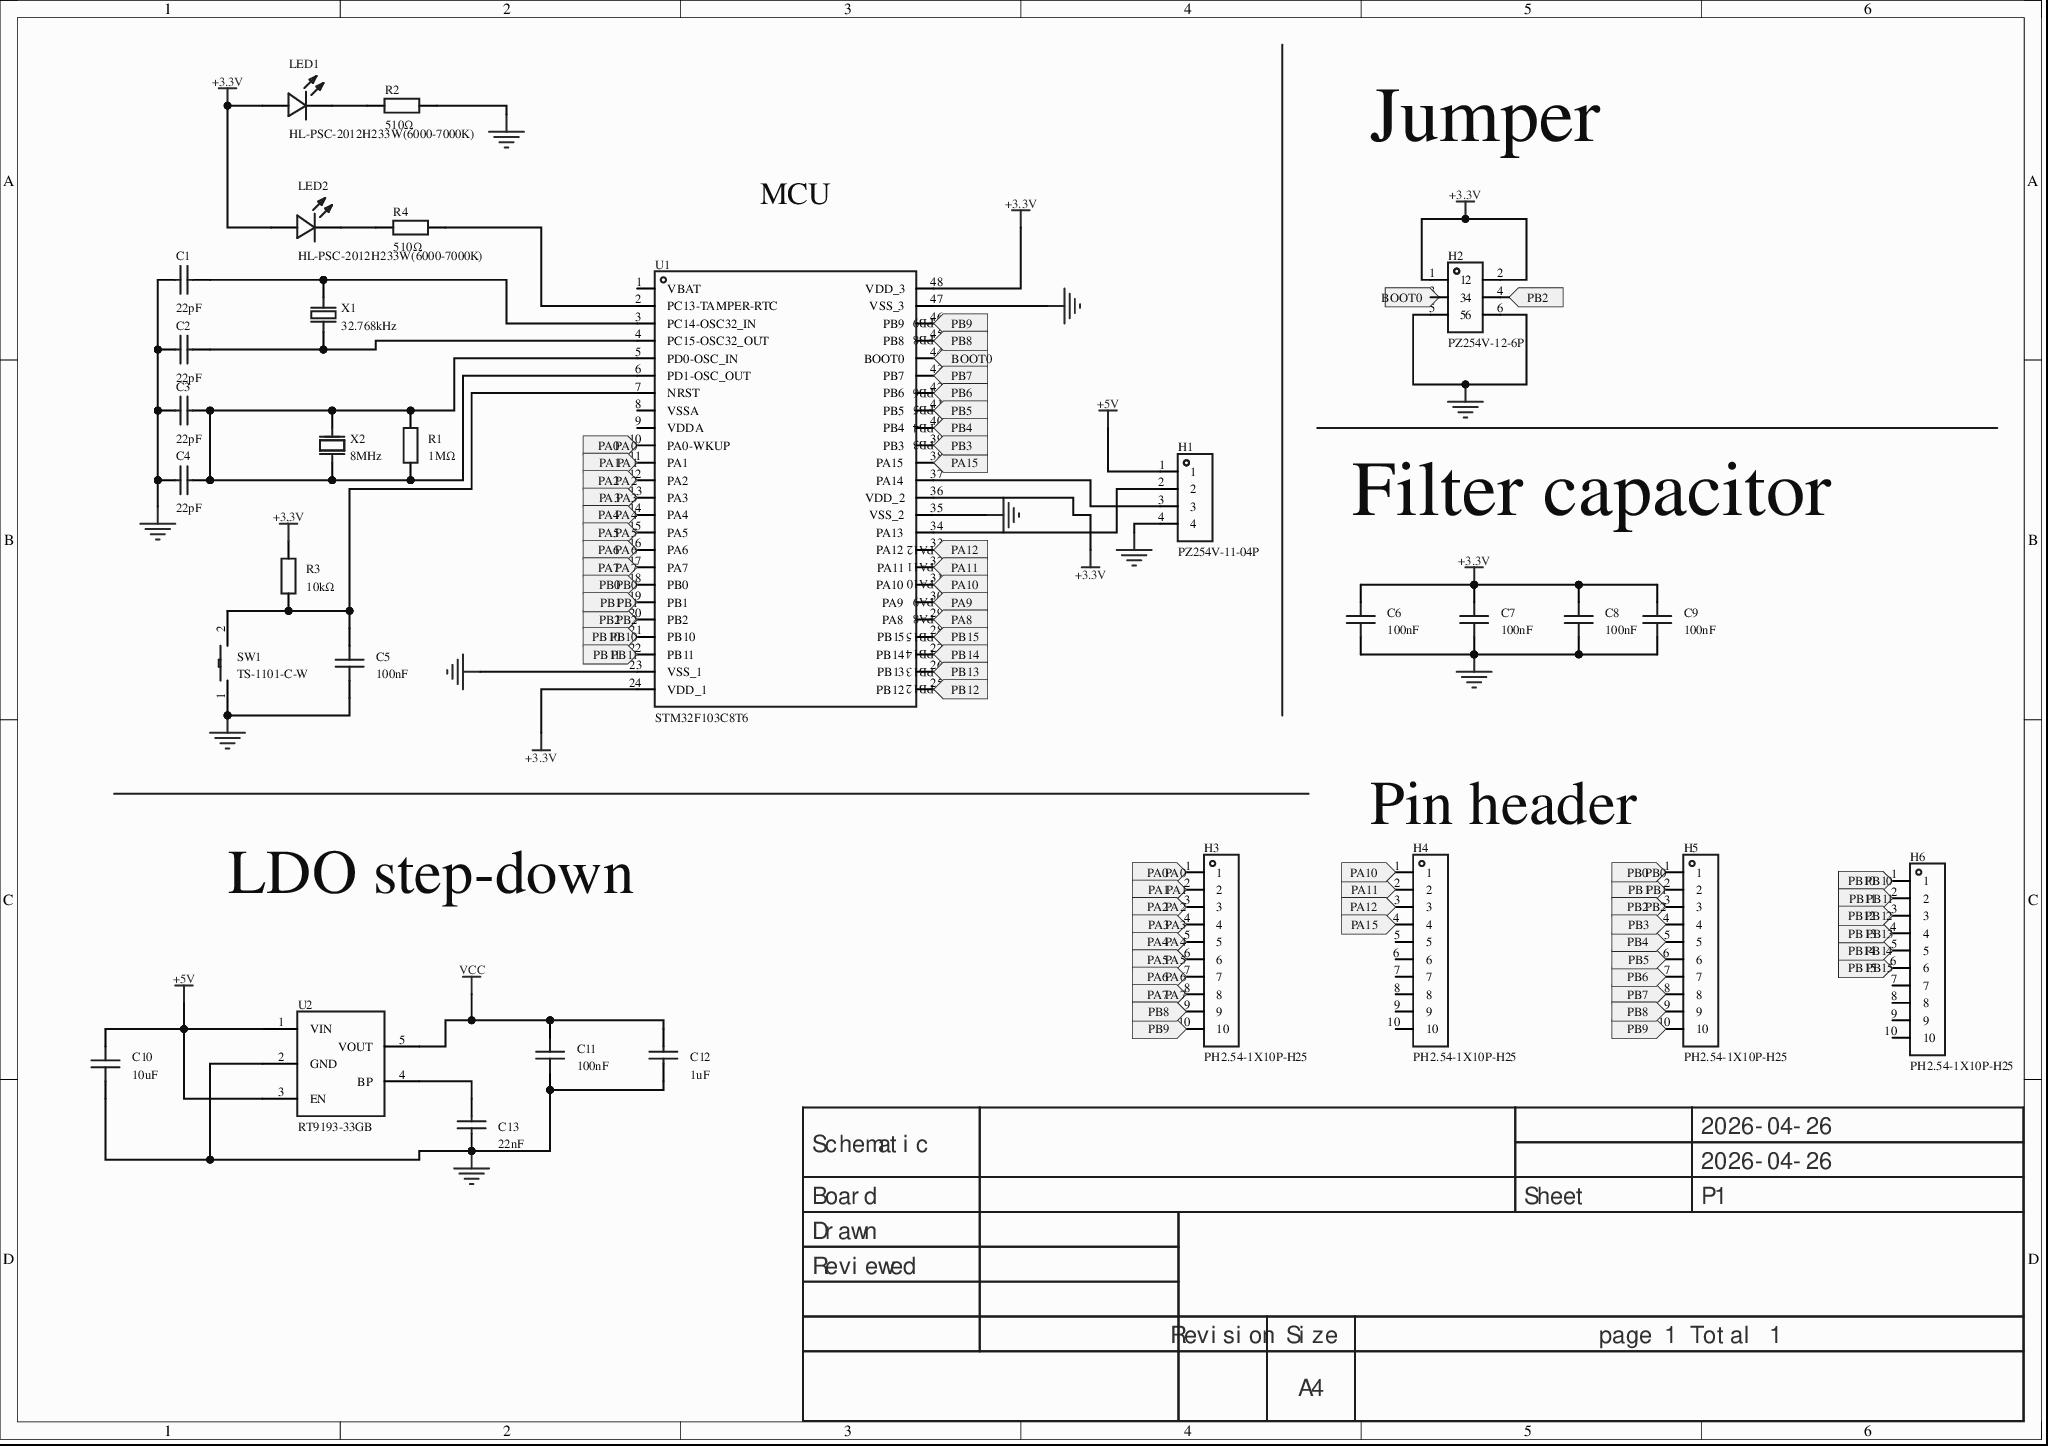
[diagram p0: MISC52025-3.schdoc]
# Altium project MISC52025-2.PrjPcb
1 sheet, 30 parts. Net scope: flat (ports and power ports of the same name join across sheets).
Board file: MISC52025.pcbdoc

## Sheet MISC52025-3.schdoc
size 297 x 209 mm; Version: V1.0; @Project Name: MISC52025; @Update Date: 2026-04-26; @Create Date: 2026-04-26; @Board Name: MISC52025; @Create Time: 15:19:25; @Page Count: 1; @Page No: 1; @Schematic Name: MISC52025; @Update Time: 15:19:25; Size: A4

### Parts
C1  22pF  [C0603]
C2  22pF  [C0603]
C3  22pF  [C0603]
C4  22pF  [C0603]
C5  100nF  [C0603]
C6  100nF  [C0603]
C7  100nF  [C0603]
C8  100nF  [C0603]
C9  100nF  [C0603]
C10  10uF  [C0603]
C11  100nF  [C0603]
C12  1uF  [C0603]
C13  22nF  [C0603]
H1  PZ254V-11-04P  [HDR-TH_4P-P2.54-V-M]
H2  PZ254V-12-6P  [HDR-TH_6P-P2.54-V-M-R2-C3-S2.54]
H3  PH2.54-1X10P-H25  [HDR-TH_10P-P2.54-V-M]
H4  PH2.54-1X10P-H25  [HDR-TH_10P-P2.54-V-M]
H5  PH2.54-1X10P-H25  [HDR-TH_10P-P2.54-V-M]
H6  PH2.54-1X10P-H25  [HDR-TH_10P-P2.54-V-M]
LED1  HL-PSC-2012H233W(6000-7000K)  [LED0805-R-RD]
LED2  HL-PSC-2012H233W(6000-7000K)  [LED0805-R-RD]
R1  1MΩ  [R0805]
R2  510Ω  [R0603]
R3  10kΩ  [R0603]
R4  510Ω  [R0603]
SW1  TS-1101-C-W  [SW-SMD_L6.0-W3.3-LS8.0_TS-1101-C-W]
U1  STM32F103C8T6  [LQFP-48_L7.0-W7.0-P0.50-LS9.0-BL]
U2  RT9193-33GB  [SOT-23-5_L3.0-W1.7-P0.95-LS2.8-BL]
X1  32.768kHz  [FC-135R_L3.2-W1.5]
X2  8MHz  [CRYSTAL-SMD_L5.0-W3.2]

### Ports
BOOT0 (in), PA0 (in), PA1 (in), PA2 (in), PA3 (in), PA4 (in), PA5 (in), PA6 (in), PA7 (in), PA8 (in), PA9 (in), PA10 (in), PA11 (in), PA12 (in), PA15 (in), PB0 (in), PB1 (in), PB2 (in), PB3 (in), PB4 (in), PB5 (in), PB6 (in), PB7 (in), PB8 (in), PB9 (in), PB10 (in), PB11 (in), PB12 (in), PB13 (in), PB14 (in), PB15 (in)

### Nets
+3,3V: R3.2
+3.3V: C6.2 C7.2 C8.2 C9.2 H2.1 H2.2 LED1.1(A) LED2.1(A) U1.24(VDD_1) U1.36(VDD_2) U1.48(VDD_3)
+5V: C10.2 H1.1 U2.1(VIN) U2.3(EN)
GND: C1.1 C2.1 C3.1 C4.1 C5.1 C6.1 C7.1 C8.1 C9.1 C10.1 C11.1 C12.1 C13.1 H1.4 H2.5 H2.6 R2.2 SW1.1 U1.23(VSS_1) U1.35(VSS_2) U1.47(VSS_3) U2.2(GND)
VCC: C11.2 C12.2 U2.5(VOUT)
PA0: H3.1 U1.10(PA0-WKUP) ; port PA0
PA1: H3.2 U1.11(PA1) ; port PA1
PA2: H3.3 U1.12(PA2) ; port PA2
PA3: H3.4 U1.13(PA3) ; port PA3
PA4: H3.5 U1.14(PA4) ; port PA4
PA5: H3.6 U1.15(PA5) ; port PA5
PA6: H3.7 U1.16(PA6) ; port PA6
PA7: H3.8 U1.17(PA7) ; port PA7
PA8: U1.29(PA8) ; port PA8
PA9: U1.30(PA9) ; port PA9
PA10: H4.1 U1.31(PA10) ; port PA10
PA11: H4.2 U1.32(PA11) ; port PA11
PA12: H4.3 U1.33(PA12) ; port PA12
PB0: H5.1 U1.18(PB0) ; port PB0
PB1: H5.2 U1.19(PB1) ; port PB1
PB2: H2.4 H5.3 U1.20(PB2) ; port PB2
PB3: H5.4 U1.39(PB3) ; port PB3
PB4: H5.5 U1.40(PB4) ; port PB4
PB5: H5.6 U1.41(PB5) ; port PB5
PB6: H5.7 U1.42(PB6) ; port PB6
PB8: H3.9 H5.9 U1.45(PB8) ; port PB8
PB9: H3.10 H5.10 U1.46(PB9) ; port PB9
PB10: H6.1 U1.21(PB10) ; port PB10
PB11: H6.2 U1.22(PB11) ; port PB11
PB12: H6.3 U1.25(PB12) ; port PB12
PB13: H6.4 U1.26(PB13) ; port PB13
PB14: H6.5 U1.27(PB14) ; port PB14
PB15: H6.6 U1.28(PB15) ; port PB15
NetC1_2: C1.2 U1.3(PC14-OSC32_IN) X1.2
NetC2_2: C2.2 U1.4(PC15-OSC32_OUT) X1.1
NetC3_2: C3.2 C4.2 R1.1 R1.2 U1.5(PD0-OSC_IN) U1.6(PD1-OSC_OUT) X2.1(OSC1) X2.2(OSC2)
NetC5_2: C5.2 R3.1 SW1.2 U1.7(NRST)
NetC13_2: C13.2 U2.4(BP)
NetH1_2: H1.2 U1.34(PA13)
NetH1_3: H1.3 U1.37(PA14)
NetH2_3: H2.3 U1.44(BOOT0) ; port BOOT0
NetH4_4: H4.4 U1.38(PA15) ; port PA15
NetH5_8: H5.8 U1.43(PB7) ; port PB7
NetLED1_2: LED1.2(C) R2.1
NetLED2_2: LED2.2(C) R4.1
NetR4_2: R4.2 U1.2(PC13-TAMPER-RTC)

Not connected (* = marked no-connect by the designer): H4 5 6 7 8 9 10; H6 7 8 9 10; U1 1(VBAT) 8(VSSA) 9(VDDA)

### Notes on the sheet
- Jumper
- MCU
- Filter capacitor
- Pin header
- LDO step-down
- 2026-04-26
- Schematic
- Board
- Sheet
- P1
- Drawn
- Reviewed
- Revision
- Size
- A4
- page 1 Total 1

### Library data of the parts
C1-C4 = CL10C220JB8NNNC: Capacitance:22pF;Tolerance:±5%;Rated voltage:50V;Temperature coefficient:C0G;; Manufacturer: SAMSUNG(三星); 3D Model: ac125912035d415993ca9572d50418b10819f05c4eef4c71ace90d822a990e87; 3D Model Transform: 62.992,31.496,0,0,0,0,0,0,0; Tolerance: ±5%; Voltage Rating: 50V; Temperature Coefficient: C0G; AddInBom: yes; ModelName: C0603_L1.6-W0.8-H0.8; Symbol: CL10C220JB8NNNC; Device: CL10C220JB8NNNC; LCSC Part Name: 22pF ±5% 50V; Supplier Part: C1653; Manufacturer Part: CL10C220JB8NNNC; Supplier Footprint: 0603; JLCPCB Part Class: Basic Part; Datasheet: https://example.com/datasheet/CL10C220JB8NNNC/2005.html; Supplier: LCSC; Value: 22pF; ConvertToPcb: yes; FootprintName: C0603
C5-C9 C11 = CC0603KRX7R9BB104: Capacitance:100nF;Tolerance:±10%;Rated voltage:50V;Temperature coefficient:X7R;; Manufacturer: YAGEO(国巨); AddInBom: yes; ModelId: ac125912035d415993ca9572d50418b10819f05c4eef4c71ace90d822a990e87; ModelName: C0603_L1.6-W0.8-H0.8; ModelTransform: 62.992,31.496,0,0,0,0,0,0,0; Tolerance: ±10%; Voltage Rating: 50V; Temperature Coefficient: X7R; Symbol: CC0603KRX7R9BB104; Device: CC0603KRX7R9BB104; LCSC Part Name: 100nF ±10% 50V; SupplierPart: C14663; ManufacturerPart: CC0603KRX7R9BB104; Supplier Footprint: 0603; JLCPCB Part Class: Basic Part; Datasheet: https://example.com/datasheet/CC0603KRX7R9BB104/15331.html; Supplier: LCSC; ConvertToPcb: yes; FootprintName: C0603; Value: 100nF
C10 = CL10A106KP8NNNC: Capacitance:10uF;Tolerance:±10%;Rated voltage:10V;Temperature coefficient:X5R;; Manufacturer: SAMSUNG(三星); AddInBom: yes; ModelId: ac125912035d415993ca9572d50418b10819f05c4eef4c71ace90d822a990e87; ModelName: C0603_L1.6-W0.8-H0.8; ModelTransform: 62.992,31.496,0,0,0,0,0,0,0; Tolerance: ±10%; Voltage Rating: 10V; Temperature Coefficient: X5R; Symbol: CL10A106KP8NNNC; Device: CL10A106KP8NNNC; LCSC Part Name: 10uF ±10% 10V; SupplierPart: C19702; ManufacturerPart: CL10A106KP8NNNC; Supplier Footprint: 0603; JLCPCB Part Class: Basic Part; Datasheet: https://example.com/datasheet/CL10A106KP8NNNC/20411.html; Supplier: LCSC; ConvertToPcb: yes; FootprintName: C0603; Value: 10uF
C12 = CL10B105KO8NNNC: Capacitance:1uF;Tolerance:±10%;Rated voltage:16V;Temperature coefficient:X7R;; Manufacturer: SAMSUNG(三星); AddInBom: yes; ModelId: ac125912035d415993ca9572d50418b10819f05c4eef4c71ace90d822a990e87; ModelName: C0603_L1.6-W0.8-H0.8; ModelTransform: 62.992,31.496,0,0,0,0,0,0,0; Tolerance: ±10%; Voltage Rating: 16V; Temperature Coefficient: X7R; Symbol: CL10B105KO8NNNC; Device: CL10B105KO8NNNC; LCSC Part Name: 1uF ±10% 16V; SupplierPart: C59782; ManufacturerPart: CL10B105KO8NNNC; Supplier Footprint: 0603; JLCPCB Part Class: Extended Part; Datasheet: https://example.com/datasheet/CL10B105KO8NNNC/60834.html; Supplier: LCSC; ConvertToPcb: yes; FootprintName: C0603; Value: 1uF
C13 = CL10B223KB8NNNC: Capacitance:22nF;Tolerance:±10%;Rated voltage:50V;Temperature coefficient:X7R;; Manufacturer: SAMSUNG(三星); AddInBom: yes; ModelId: ac125912035d415993ca9572d50418b10819f05c4eef4c71ace90d822a990e87; ModelName: C0603_L1.6-W0.8-H0.8; ModelTransform: 62.992,31.496,0,0,0,0,0,0,0; Tolerance: ±10%; Voltage Rating: 50V; Temperature Coefficient: X7R; Symbol: CL10B223KB8NNNC; Device: CL10B223KB8NNNC; LCSC Part Name: 22nF ±10% 50V; SupplierPart: C21122; ManufacturerPart: CL10B223KB8NNNC; Supplier Footprint: 0603; JLCPCB Part Class: Basic Part; Datasheet: https://example.com/datasheet/CL10B223KB8NNNC/21834.html; Supplier: LCSC; ConvertToPcb: yes; FootprintName: C0603; Value: 22nF
H1 = PZ254V-11-04P: Pin structure:1x4P;Pitch:2.54mm;Row spacing:-;Round/square pin:Square;Mounting:Through-hole;Rows:Single row;Total pins:4P;Rated current:3A;Rated voltage:250V;Mating pin length:6mm;Housing height:2.5mm;Termination pin length:3mm;Contact material:-;Operating temperature:-40℃~+105℃;Colour:Black;; Manufacturer: XFCN(兴飞); Symbol: PZ254V-11-04P_C2691448; AddInBom: yes; ModelId: 112f4d05e8d64e99ab9a333894bea4f90819f05c4eef4c71ace90d822a990e87; ModelName: HDR-TH_4P-P2.54-M-LI-1X4P; ModelTransform: 399.999,104.7242,0,0,0,0,0,0,-118.11; Pin Structure: 1x4P; Pitch: 2.54mm; Circluar Pins/Square Pins: Square; Current Rating: 3A; Voltage Rating (Max): 250V; Device: PZ254V-11-04P; LCSC Part Name: 1x4P 间距:2.54mm 方针 直插; SupplierPart: C2691448; ManufacturerPart: PZ254V-11-04P; Supplier Footprint: 插件,P=2.54mm; JLCPCB Part Class: Extended Part; Datasheet: https://example.com/datasheet/PZ254V-11-04P/2801085.html; Supplier: LCSC; ConvertToPcb: yes; FootprintName: HDR-TH_4P-P2.54-V-M; Row Spacing: -; Mounting Type: Through-hole; Number of Rows: Single row; Number of Pins: 4P; Length of Mating Pin: 6mm; Insulation Height: 2.5mm; Length of End Connection Pin: 3mm; Contact Material: -; Operating Temperature: -40℃~+105℃; Color: Black
H2 = PZ254V-12-6P: Pin structure:2x3P;Pitch:2.54mm;Row spacing:2.54mm;Round/square pin:Square;Mounting type:Through-hole;Rows:Dual row;Total pins:6P;Rated current:-;Rated voltage:-;Mating pin length:6mm;Housing height:2.5mm;Termination pin length:3mm;Contact material:Brass;Contact plating:-;Operating temperature range:-40℃~+105℃;Colour:Black;; Manufacturer: XFCN(兴飞); AddInBom: yes; ModelId: e22692306cbd4b5c8488f4142eed6b9c0819f05c4eef4c71ace90d822a990e87; ModelTransform: 300.3931,200,0,0,0,0,0,0,-118.11; Pin Structure: 2x3P; Pitch: 2.54mm; Circluar Pins/Square Pins: Square; Symbol: PZ254V-12-6P; Device: PZ254V-12-6P; LCSC Part Name: 间距:2.54mm 2x3P 直插 方针; SupplierPart: C492420; ManufacturerPart: PZ254V-12-6P; Supplier Footprint: 插件,P=2.54mm; JLCPCB Part Class: Extended Part; Datasheet: https://example.com/upload/public/pdf/source/20200309/C492420_BAECB307B001054C09D200388220EAE6.pdf; Supplier: LCSC; ConvertToPcb: yes; FootprintName: HDR-TH_6P-P2.54-V-M-R2-C3-S2.54; ModelName: HDR-TH_6P-P2.54-V-M-R2-C3-S2.54; Row Spacing: 2.54mm; Mounting Type: Through-hole; Number of Rows: Dual row; Number of Pins: 6P; Current Rating (Max): -; Voltage Rating (Max): -; Length of Mating Pin: 6mm; Insulation Height: 2.5mm; Length of End Connection Pin: 3mm; Contact Material: Brass; Contact Plating: -; Operating Temperature Range: -40℃~+105℃; Color: Black
H3-H6 = PH2.54-1X10P-H25: Pin structure:1x10P;Pitch:2.54mm;Row spacing:-;Round/square pin:Square;Mounting:Through-hole;Rows:Single row;Total pins:10P;Rated current:3A;Rated voltage:-;Mating pin length:6mm;Housing height:2.5mm;Termination pin length:3mm;Contact material:Brass;Contact plating:Gold;Operating temperature:-40℃~+105℃;Colour:Black;; Manufacturer: JXTCONN(聚兴泰); AddInBom: yes; ModelId: 10f3d1cea59e4bb4ba116af9f09c2b9b0819f05c4eef4c71ace90d822a990e87; ModelName: HDR2.54-M-LI-1X10P; ModelTransform: 999.99796,100,0,0,0,0,0,0,-118.11; Pin Structure: 1x10P; Pitch: 2.54mm; Circluar Pins/Square Pins: Square; Current Rating: 3A; Symbol: PH2.54-1X10P-H25; Device: PH2.54-1X10P-H25; LCSC Part Name: 1x10P 间距:2.54mm 方针 直插; SupplierPart: C42431810; ManufacturerPart: PH2.54-1X10P-H25; Supplier Footprint: 插件,P=2.54mm; JLCPCB Part Class: Extended Part; Datasheet: https://example.com/datasheet/PH2.54-1X10P-H25/44458940.html; Supplier: LCSC; ConvertToPcb: yes; FootprintName: HDR-TH_10P-P2.54-V-M; Row Spacing: -; Mounting Type: Through-hole; Number of Rows: Single row; Number of Pins: 10P; Voltage Rating (Max): -; Length of Mating Pin: 6mm; Insulation Height: 2.5mm; Length of End Connection Pin: 3mm; Contact Material: Brass; Contact Plating: Gold; Operating Temperature: -40℃~+105℃; Color: Black
LED1 LED2 = HL-PSC-2012H233W(6000-7000K): Lamp base type:-;Emitting colour:White;Forward voltage (Vf):3.4V;Power:102mW;Forward current:20mA;Wavelength:-;Diode configuration:Single diode;Lens colour:Frosted yellow lens;Colour temperature:6000K~7000K;Luminous intensity:1.4cd;Viewing angle:140°;Tape packaging:Top mount;Operating temperature:-40℃~+85℃;; Manufacturer: HONGLITRONIC(鸿利光电); AddInBom: yes; ModelId: 6ccd75a2b5134d6ab756ecf3c14a72900819f05c4eef4c71ace90d822a990e87; ModelName: LED0805-RD; ModelTransform: 79.527,49.2125,0,0,0,0,0,0,0; Illumination Color: White; Voltage - Forward(Vf): 3.4V; Power(Watts): 102mW; Forward Current: 20mA; Luminous Intensity: 1.4cd; Viewing Angle: 140°; Symbol: HL-PSC-2012H233W(6000-7000K); Device: HL-PSC-2012H233W(6000-7000K); LCSC Part Name: 白色; SupplierPart: C219231; ManufacturerPart: HL-PSC-2012H233W(6000-7000K); Supplier Footprint: 0805; JLCPCB Part Class: Extended Part; Datasheet: https://example.com/datasheet/HL-PSC-2012H233W(6000-7000K)/220090.html; Supplier: LCSC; ConvertToPcb: yes; FootprintName: LED0805-R-RD; Lamp Holder Type: -; Wavelength - Dominant: -; Peak Wavelength: -; Diode Configuration: Single diode; Lens Color: Frosted yellow lens; Color Temperature: 6000K~7000K; Mounting Style: Top mount; Operating Temperature: -40℃~+85℃
R1 = 0805W8F1004T5E: Resistor type:Thick film resistor;Resistance:1MΩ;Tolerance:±1%;Power:125mW;Max working voltage:150V;Temperature coefficient:±100ppm/℃;; Manufacturer: UNI-ROYAL(厚声); AddInBom: yes; ModelId: 37a81e68749a4138bd2dfa6897b24b850819f05c4eef4c71ace90d822a990e87; ModelName: R0805_L2.0-W1.3-H0.6; ModelTransform: 78.74,51.181,0,0,0,0,0,-0.0005,0; Tolerance: ±1%; Power(Watts): 125mW; Overload Voltage (Max): 150V; Symbol: 0805W8F1004T5E; Device: 0805W8F1004T5E; LCSC Part Name: 1MΩ ±1% 125mW 厚膜电阻; SupplierPart: C17514; ManufacturerPart: 0805W8F1004T5E; Supplier Footprint: 0805; JLCPCB Part Class: Basic Part; Datasheet: https://example.com/upload/public/pdf/source/20200306/C422600_1E6D84923E4A46A82E41ADD87F860B5C.pdf; Supplier: LCSC; ConvertToPcb: yes; FootprintName: R0805; Type: Thick film resistor; Value: 1MΩ; Temperature Coefficient: ±100ppm/℃; Operating Temperature Range: -55℃~+155℃
R2 R4 = 0603WAF5100T5E: Resistor type:Thick film resistor;Resistance:510Ω;Tolerance:±1%;Power:100mW;Working voltage:75V;Temperature coefficient:±100ppm/℃;; Manufacturer: UNI-ROYAL(厚声); AddInBom: yes; ModelId: fc143cca1e79419f9cd78b61e9279f080819f05c4eef4c71ace90d822a990e87; ModelTransform: 31.8897,63.7794,0,90,0,0,0,0,0; Tolerance: ±1%; Power(Watts): 100mW; Voltage-Supply(Max): 75V; Symbol: 0603WAF5100T5E; Device: 0603WAF5100T5E; LCSC Part Name: 510Ω ±1% 100mW 厚膜电阻; SupplierPart: C23193; ManufacturerPart: 0603WAF5100T5E; Supplier Footprint: 0603; JLCPCB Part Class: Basic Part; Datasheet: https://example.com/datasheet/0603WAF5100T5E/23920.html; Supplier: LCSC; ConvertToPcb: yes; FootprintName: R0603; ModelName: R0603; Type: Thick film resistor; Value: 510Ω; Temperature Coefficient: ±100ppm/℃; Operating Temperature: -55℃~+155℃
R3 = 0603WAF1002T5E: Resistor type:Thick film resistor;Resistance:10kΩ;Tolerance:±1%;Power:100mW;Working voltage:75V;Temperature coefficient:±100ppm/℃;; Manufacturer: UNI-ROYAL(厚声); AddInBom: yes; ModelId: fc143cca1e79419f9cd78b61e9279f080819f05c4eef4c71ace90d822a990e87; ModelTransform: 31.8897,63.7794,0,90,0,0,0,0,0; Tolerance: ±1%; Power(Watts): 100mW; Voltage-Supply(Max): 75V; Symbol: 0603WAF1002T5E; Device: 0603WAF1002T5E; LCSC Part Name: 厚膜电阻 10kΩ ±1% 100mW; SupplierPart: C25804; ManufacturerPart: 0603WAF1002T5E; Supplier Footprint: 0603; JLCPCB Part Class: Basic Part; Datasheet: https://example.com/datasheet/0603WAF1002T5E/26547.html; Supplier: LCSC; ConvertToPcb: yes; FootprintName: R0603; ModelName: R0603; Type: Thick film resistor; Value: 10kΩ; Temperature Coefficient: ±100ppm/℃; Operating Temperature: -55℃~+155℃
SW1 = TS-1101-C-W: Circuit structure:SPST;Button shape:Rectangular button;Actuating force:2.6N;Mounting:Upright SMD;Switch length:6mm;Switch width:3.6mm;Switch height:2.5mm;Bracket:Without bracket;Contact current:50mA;Rated voltage:12V;Lamp:None;Life:5万 cycles;; Manufacturer: XKB Connection(中国星坤); AddInBom: yes; ModelId: 0fd6340cfb7d45bfbbb5f8576d023f850819f05c4eef4c71ace90d822a990e87; ModelTransform: 315.232,145.669,0,0,0,0,0,0,0; Circuit: SPST; Operating Force: 2.6N; Switch Height: 2.5mm; Contact Current: 50mA; Voltage Rating: 12V; With Lamp: None; Symbol: TS-1101-C-W; Device: TS-1101-C-W; LCSC Part Name: 6*3.6*2.5mm 立贴 轻触开关; SupplierPart: C318938; ManufacturerPart: TS-1101-C-W; Supplier Footprint: SMD,6x3.6mm; JLCPCB Part Class: Extended Part; Datasheet: https://example.com/datasheet/TS-1101-C-W/300030.html; Supplier: LCSC; ConvertToPcb: yes; FootprintName: SW-SMD_L6.0-W3.3-LS8.0_TS-1101-C-W; ModelName: SW-SMD_L6.0-W3.3-LS8.0_TS-1101-C-W; Actuator Style: Rectangular button; Mounting Type: Upright SMD; Length: 6mm; Width: 3.6mm; with Bracket: Without bracket; Actuator/Cap Color: -; IP Rating: -; Termination Style: -; Life: 5万 cycles; Operating Temperature: -30℃~+85℃
U1 = STM32F103C8T6: CPU core:ARM-M3;CPU max frequency:72MHz;Application field:-;; Manufacturer: ST(意法半导体); 3D Model: 093be70396ff421eb2cdb946d5311efc0819f05c4eef4c71ace90d822a990e87; 3D Model Transform: 354.331,354.331,0,0,0,0,0,0,0; CPU Core: ARM-M3; CPU Maximum Speed: 72MHz; Program Storage Size: 64KB; Program Memory Type: FLASH; Number of I/O: 37; ADC (Bit): 12bit; Voltage - Supply: 2V~3.6V; AddInBom: yes; ModelName: LQFP-48_L7.0-W7.0-H1.4-LS9.0-P0.50; Symbol: STM32F103C8T6; Device: STM32F103C8T6; LCSC Part Name: 主流增强型ARM Cortex-M3 MCU，具有64 KB Flash、72 MHz CPU、电机控制、USB和CAN; Supplier Part: C8734; Manufacturer Part: STM32F103C8T6; Supplier Footprint: LQFP-48(7x7); JLCPCB Part Class: Extended Part; Datasheet: https://example.com/datasheet/STM32F103C8T6/9243.html; Supplier: LCSC; Applications: -; ConvertToPcb: yes; FootprintName: LQFP-48_L7.0-W7.0-P0.50-LS9.0-BL
U2 = RT9193-33GB: Output type:Fixed;Working voltage:5.5V;Output voltage:3.3V;Output current:300mA;Power supply ripple rejection (PSRR):-50dB@(10kHz);Output polarity:Positive;; Manufacturer: RICHTEK(立锜); AddInBom: yes; ModelId: 0a2a1b8f50944f73965918ad6e5fe1670819f05c4eef4c71ace90d822a990e87; ModelName: SOT-23-5_L2.9-W1.6-H1.1-LS2.8-P0.95; ModelTransform: 118.60433,114.173,0,90,0,0,0.0005,0.0005,0; Output Type: Fixed; Voltage - Supply: 5.5V; Output Voltage: 3.3V; Output Current: 300mA; Voltage Dropout: 220mV@(300mA); standby current: 90uA; Noise: 100uVrms; Number of Outputs: 1; Symbol: RT9193-33GB; Device: RT9193-33GB; LCSC Part Name: 输入5.5V 输出3.3V 300mA; SupplierPart: C15651; ManufacturerPart: RT9193-33GB; Supplier Footprint: SOT-23-5; JLCPCB Part Class: Extended Part; Datasheet: https://example.com/datasheet/RT9193-33GB/16332.html; Supplier: LCSC; ConvertToPcb: yes; FootprintName: SOT-23-5_L3.0-W1.7-P0.95-LS2.8-BL; Power Supply Rejection Ratio (PSRR): -50dB@(10kHz); Features: Overcurrent protection; enable; overtemperature protection; Operating Temperature: -40℃~+125℃@(Tj); Output Configuration: Positive
X1 = Q13FC13500004_C32346: Crystal type:SMD crystal;Frequency:32.768kHz;Room-temp tolerance:±20ppm;Load capacitance:12.5pF;; Manufacturer: EPSON(爱普生); Symbol: Q13FC1350000400; AddInBom: yes; ModelId: 751105e878f044059ef0ee72de95f96e0819f05c4eef4c71ace90d822a990e87; ModelTransform: 125.984,59.055,0,0,0,0,0,0,0; Normal temperature Frequency Tolerance: ±20ppm; Load Capacitance: 12.5pF; Equivalent Series Resistance(ESR): 70kΩ; Device: Q13FC13500004_C32346; LCSC Part Name: 32.768kHz ±20ppm 12.5pF; SupplierPart: C32346; ManufacturerPart: Q13FC13500004; Supplier Footprint: SMD3215-2P; JLCPCB Part Class: Basic Part; Datasheet: https://example.com/datasheet/Q13FC13500004/33310.html; Supplier: LCSC; ConvertToPcb: yes; FootprintName: FC-135R_L3.2-W1.5; ModelName: FC-135R_L3.2-W1.5; Type: SMD crystal; Value: 32.768kHz; Operating Temperature: -40℃~+85℃
X2 = X50328MSB2GI: Crystal type:SMD crystal;Frequency:8MHz;Room-temp tolerance:±10ppm;Load capacitance:20pF;Frequency stability:±20ppm;; Manufacturer: YXC(扬兴晶振); AddInBom: yes; ModelId: d7c39c66443246ff83c2003c1e1eb6f10819f05c4eef4c71ace90d822a990e87; ModelTransform: 196.85,125.984,0,0,0,0,0,0,0; Normal temperature Frequency Tolerance: ±10ppm; Load Capacitance: 20pF; Frequency Stability: ±20ppm; Symbol: X50328MSB2GI; Device: X50328MSB2GI; LCSC Part Name: YSX530GA 8MHZ 2P 5032 20PF ±10PPM -40~85℃ (±20PPM); SupplierPart: C115962; ManufacturerPart: X50328MSB2GI; Supplier Footprint: SMD5032-2P; JLCPCB Part Class: Basic Part; Datasheet: https://example.com/datasheet/X50328MSB2GI/117214.html; Supplier: LCSC; ConvertToPcb: yes; FootprintName: CRYSTAL-SMD_L5.0-W3.2; ModelName: CRYSTAL-SMD_L5.0-W3.2; Type: SMD crystal; Value: 8MHz; Operating Temperature: -40℃~+85℃